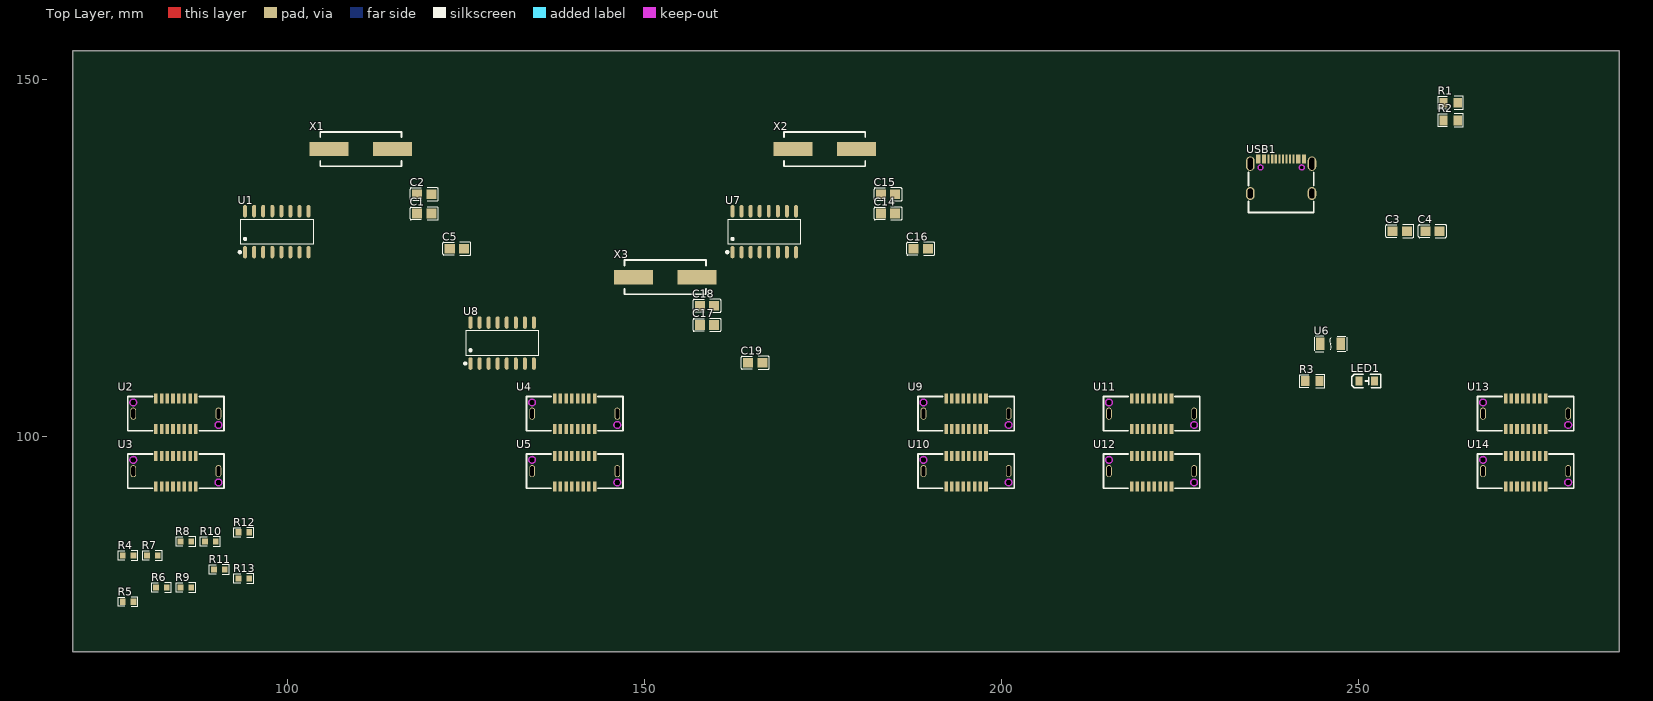
[diagram p0: Top Layer view]
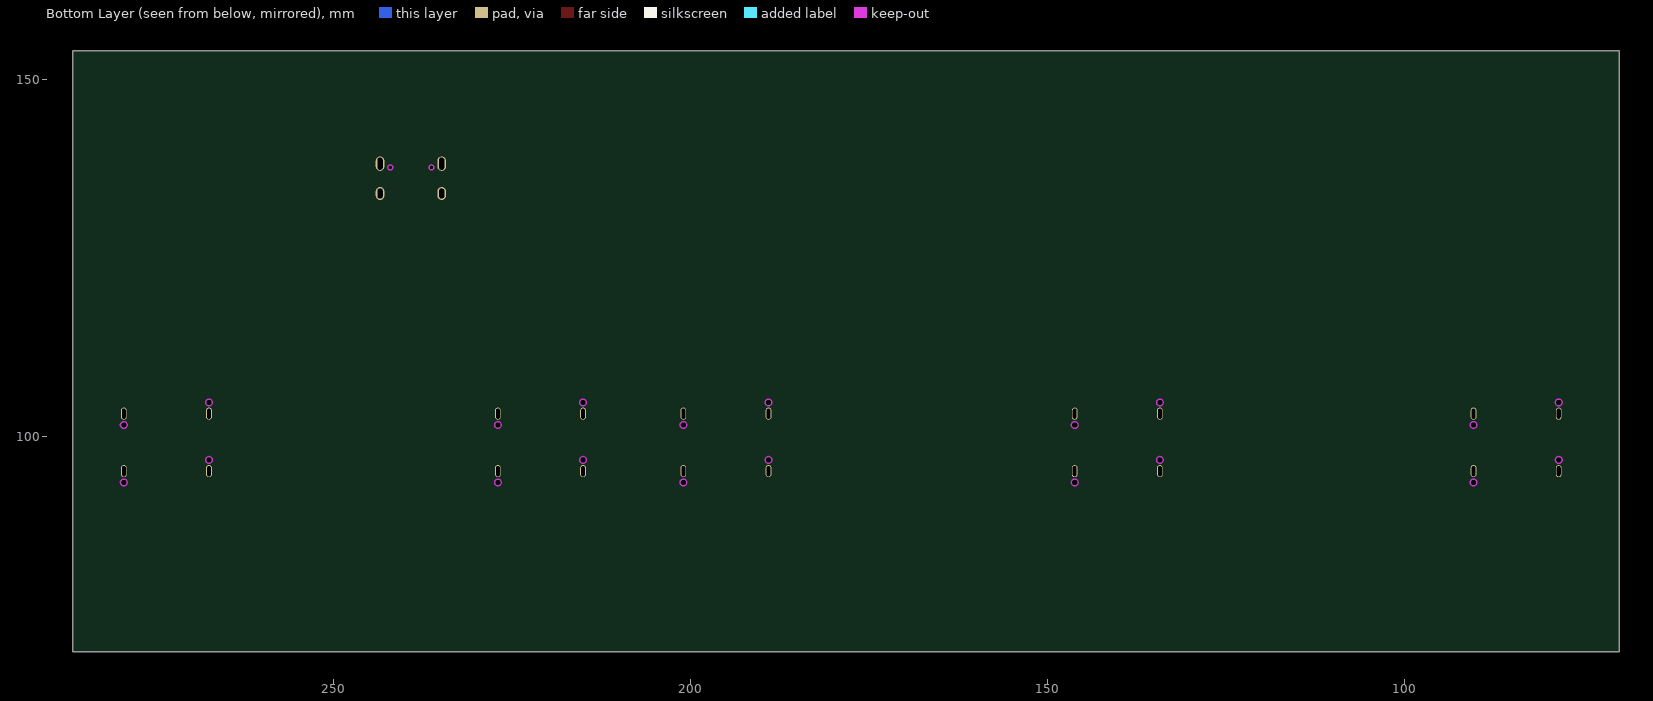
[diagram p1: Bottom Layer view, seen from below]
# Altium PCB MISC51596.pcbdoc
Units mm, origin at the board's own origin, x right, y up, seen from the top; angles counter-clockwise.
Board outline 216.76 x 84.23 mm, 2 copper layers (Top Layer, Bottom Layer), stack 1.58 mm thick; 43 components, 45 nets, 306 pads, 0 vias.

## Layer stack, top to bottom
Top Solder Mask Layer: solder mask 0.01, Dk 3.3
Top Layer: signal copper 0.035
Dielectric1: surface 1.51, FR4, Dk 4.5
Bottom Layer: signal copper 0.035
Bottom Solder Mask Layer: solder mask 0.01, Dk 3.3

## Board outline
286.61,69.85 69.85,69.85 69.85,154.083 286.61,154.083

## Design rules (kind name [scope] priority, off if disabled: settings)
BoardOutlineClearance copperThickness2oz_1 [All] p2 off: genericclearance=0.203 ignorepadtopadclearanceinfootprint=FALSE except(0: Arc-SplitContinuation Track-SplitContinuation SMDPad-SplitContinuation THPad-SplitContinuation Via-SplitContinuation Fill-SplitContinuation Region-SplitContinuation Poly-SplitContinuation Text-SplitContinuation Hole-SplitContinuation; 0.152: SMDPad-CutoutEdge THPad-CutoutEdge Via-CutoutEdge Fill-CutoutEdge Region-CutoutEdge Text-CutoutEdge Hole-CutoutEdge; 0.254: Poly-OutlineEdge Poly-CutoutEdge; 0.3: Arc-OutlineEdge Track-OutlineEdge SMDPad-OutlineEdge THPad-OutlineEdge Via-OutlineEdge Fill-OutlineEdge Region-OutlineEdge Text-OutlineEdge Hole-OutlineEdge Arc-CutoutEdge Track-CutoutEdge)
BoardOutlineClearance Plane_innerPlane_1 [All] p4 off: genericclearance=0.102 ignorepadtopadclearanceinfootprint=FALSE except(0: Arc-SplitContinuation Track-SplitContinuation SMDPad-SplitContinuation THPad-SplitContinuation Via-SplitContinuation Fill-SplitContinuation Region-SplitContinuation Poly-SplitContinuation Text-SplitContinuation Hole-SplitContinuation; 0.152: SMDPad-CutoutEdge THPad-CutoutEdge Via-CutoutEdge Fill-CutoutEdge Region-CutoutEdge Text-CutoutEdge Hole-CutoutEdge; 0.254: Poly-OutlineEdge Poly-CutoutEdge; 0.3: Arc-OutlineEdge Track-OutlineEdge SMDPad-OutlineEdge THPad-OutlineEdge Via-OutlineEdge Fill-OutlineEdge Region-OutlineEdge Text-OutlineEdge Hole-OutlineEdge Arc-CutoutEdge Track-CutoutEdge)
BoardOutlineClearance Copper_copperRegion_1 [All] p6 off: genericclearance=0.102 ignorepadtopadclearanceinfootprint=FALSE except(0: Arc-SplitContinuation Track-SplitContinuation SMDPad-SplitContinuation THPad-SplitContinuation Via-SplitContinuation Fill-SplitContinuation Region-SplitContinuation Poly-SplitContinuation Text-SplitContinuation Hole-SplitContinuation; 0.152: SMDPad-CutoutEdge THPad-CutoutEdge Via-CutoutEdge Fill-CutoutEdge Region-CutoutEdge Text-CutoutEdge Hole-CutoutEdge; 0.254: Poly-OutlineEdge Poly-CutoutEdge; 0.3: Arc-OutlineEdge Track-OutlineEdge SMDPad-OutlineEdge THPad-OutlineEdge Via-OutlineEdge Fill-OutlineEdge Region-OutlineEdge Text-OutlineEdge Hole-OutlineEdge Arc-CutoutEdge Track-CutoutEdge)
BoardOutlineClearance copperThickness1oz_1 [All] p8: genericclearance=0.102 ignorepadtopadclearanceinfootprint=FALSE except(0: Arc-SplitContinuation Track-SplitContinuation SMDPad-SplitContinuation THPad-SplitContinuation Via-SplitContinuation Fill-SplitContinuation Region-SplitContinuation Poly-SplitContinuation Text-SplitContinuation Hole-SplitContinuation; 0.152: SMDPad-CutoutEdge THPad-CutoutEdge Via-CutoutEdge Fill-CutoutEdge Region-CutoutEdge Text-CutoutEdge Hole-CutoutEdge; 0.254: Poly-OutlineEdge Poly-CutoutEdge; 0.3: Arc-OutlineEdge Track-OutlineEdge SMDPad-OutlineEdge THPad-OutlineEdge Via-OutlineEdge Fill-OutlineEdge Region-OutlineEdge Text-OutlineEdge Hole-OutlineEdge Arc-CutoutEdge Track-CutoutEdge)
Clearance copperThickness2oz [All] p1 off: gap=0.203 ignorepadtopadclearanceinfootprint=FALSE except(0.152: SMDPad-Track SMDPad-SMDPad THPad-Track SMDPad-THPad THPad-THPad Track-Via SMDPad-Via THPad-Via Via-Via Fill-Track Region-Track Fill-SMDPad Region-SMDPad Fill-THPad Region-THPad Fill-Via Region-Via Fill-Fill Fill-Region Region-Region Arc-Track Arc-SMDPad Arc-THPad Arc-Via Fill-Arc Region-Arc Arc-Arc Text-Track SMDPad-Text Text-THPad Text-Via Fill-Text Region-Text Arc-Text Text-Text Hole-Track Hole-SMDPad Hole-THPad Hole-Via Fill-Hole Region-Hole Hole-Arc Hole-Text; 0.254: Poly-Track Poly-SMDPad Poly-THPad Poly-Via Poly-Fill Poly-Region Poly-Poly Poly-Arc Poly-Text Poly-Hole)
Clearance Plane_innerPlane [All] p3 off: gap=0.102 ignorepadtopadclearanceinfootprint=FALSE except(0.152: SMDPad-Track SMDPad-SMDPad THPad-Track SMDPad-THPad THPad-THPad Track-Via SMDPad-Via THPad-Via Via-Via Fill-Track Region-Track Fill-SMDPad Region-SMDPad Fill-THPad Region-THPad Fill-Via Region-Via Fill-Fill Fill-Region Region-Region Arc-Track Arc-SMDPad Arc-THPad Arc-Via Fill-Arc Region-Arc Arc-Arc Text-Track SMDPad-Text Text-THPad Text-Via Fill-Text Region-Text Arc-Text Text-Text Hole-Track Hole-SMDPad Hole-THPad Hole-Via Fill-Hole Region-Hole Hole-Arc Hole-Text; 0.254: Poly-Track Poly-SMDPad Poly-THPad Poly-Via Poly-Fill Poly-Region Poly-Poly Poly-Arc Poly-Text Poly-Hole)
Clearance Copper_copperRegion [All] p5 off: gap=0.102 ignorepadtopadclearanceinfootprint=FALSE except(0.152: SMDPad-Track SMDPad-SMDPad THPad-Track SMDPad-THPad THPad-THPad Track-Via SMDPad-Via THPad-Via Via-Via Fill-Track Region-Track Fill-SMDPad Region-SMDPad Fill-THPad Region-THPad Fill-Via Region-Via Fill-Fill Fill-Region Region-Region Arc-Track Arc-SMDPad Arc-THPad Arc-Via Fill-Arc Region-Arc Arc-Arc Text-Track SMDPad-Text Text-THPad Text-Via Fill-Text Region-Text Arc-Text Text-Text Hole-Track Hole-SMDPad Hole-THPad Hole-Via Fill-Hole Region-Hole Hole-Arc Hole-Text; 0.254: Poly-Track Poly-SMDPad Poly-THPad Poly-Via Poly-Fill Poly-Region Poly-Poly Poly-Arc Poly-Text Poly-Hole)
Clearance copperThickness1oz [All] p7: gap=0.102 ignorepadtopadclearanceinfootprint=FALSE except(0.152: SMDPad-Track SMDPad-SMDPad THPad-Track SMDPad-THPad THPad-THPad Track-Via SMDPad-Via THPad-Via Via-Via Fill-Track Region-Track Fill-SMDPad Region-SMDPad Fill-THPad Region-THPad Fill-Via Region-Via Fill-Fill Fill-Region Region-Region Arc-Track Arc-SMDPad Arc-THPad Arc-Via Fill-Arc Region-Arc Arc-Arc Text-Track SMDPad-Text Text-THPad Text-Via Fill-Text Region-Text Arc-Text Text-Text Hole-Track Hole-SMDPad Hole-THPad Hole-Via Fill-Hole Region-Hole Hole-Arc Hole-Text; 0.254: Poly-Track Poly-SMDPad Poly-THPad Poly-Via Poly-Fill Poly-Region Poly-Poly Poly-Arc Poly-Text Poly-Hole)
DiffPairsRouting differentialPair [All] p1: maxlimit=0.152 minlimit=0.152 mostfreqgap=0.152 toplayer_minwidth=0.127 toplayer_prefwidth=0.254 toplayer_maxwidth=2.54 toplayer_mingap=0.152 toplayer_prefgap=0.152 toplayer_maxgap=0.152 bottomlayer_minwidth=0.127 bottomlayer_prefwidth=0.254 bottomlayer_maxwidth=2.54 bottomlayer_mingap=0.152 bottomlayer_prefgap=0.152 bottomlayer_maxgap=0.152 maxuncoupledlength=0.127
HoleToHoleClearance otherClearance [All] p1: gap=0.3 allowstackedmicrovias=TRUE
Length netLength [All] p1: minlimit=0 maxlimit=0
PasteMaskExpansion pasteMaskExpansion [All] p1: expansion=0
PlaneConnect innerPlane [All] p1: planeconnectstyle=Relief reliefexpansion=0.508 reliefentries=4 reliefconductorwidth=0.254 reliefairgap=0.254
PolygonConnect copperRegion [All] p1: connectstyle=Relief reliefconductorwidth=0.254 reliefentries=4 polygonreliefangle="90 Angle" airgapwidth=0.254 via.connectstyle=Relief via.reliefconductorwidth=0.254 via.reliefentries=4 via.polygonreliefangle="90 Angle" via.airgapwidth=0.254
RoutingVias viaSize [All] p1: holewidth=0.305 width=0.61 viastyle="Through Hole" minholewidth=0.3 minwidth=0.5 maxholewidth=6.299 maxwidth=10
SolderMaskExpansion solderMaskExpansion [IsVia] p1: expansion=-25.4 istentingtop=TRUE
SolderMaskExpansion solderMaskExpansion [All] p2: expansion=0.051 istentingtop=FALSE
Width copperThickness2oz_2 [All] p1 off: maxlimit=2.54 minlimit=0.203 preferedwidth=0.254
Width copperThickness1oz_2 [All] p2: maxlimit=2.54 minlimit=0.127 preferedwidth=0.254

## Components (designator, comment, footprint, x,y, rotation, side; value= is the part's Value field where it differs from the comment)
C1 "100nF" C0805 119.111,131.274 r0 top
C2 "100nF" C0805 119.111,133.959 r0 top
C3 "10UF" C0805 255.864,128.815 r0 top
C4 "0.1UF" C0805 260.443,128.815 r0 top
C5 "0.1UF" C0805 123.69,126.355 r0 top
C14 "100nF" C0805 184.127,131.274 r0 top
C15 "100nF" C0805 184.127,133.959 r0 top
C16 "0.1UF" C0805 188.706,126.355 r0 top
C17 "100nF" C0805 158.75,115.657 r0 top
C18 "100nF" C0805 158.75,118.342 r0 top
C19 "0.1UF" C0805 165.497,110.36 r0 top
LED1 "" LED_0805 251.267,107.788 r0 top
R1 "5.1K" R0805 262.983,146.816 r0 top
R2 "5.1K" R0805 262.983,144.329 r0 top
R3 "2K" R0805 243.605,107.788 r0 top
R4 "10K" R0603 77.585,83.348 r0 top
R5 "10K" R0603 77.585,76.861 r0 top
R6 "10K" R0603 82.278,78.834 r0 top
R7 "10K" R0603 81.008,83.348 r0 top
R8 "10K" R0603 85.7,85.321 r0 top
R9 "10K" R0603 85.7,78.834 r0 top
R10 "10K" R0603 89.123,85.321 r0 top
R11 "10K" R0603 90.393,81.374 r0 top
R12 "10K" R0603 93.815,86.591 r0 top
R13 "10K" R0603 93.815,80.104 r0 top
U1 "SL2.1A" SOP-16_L10.0-W3.9-P1.27-LS6.0-BL 98.441,128.734 r0 top
U2 "EZ-USBC-1143C" USB-SMD_EZ-USBC-1143C 84.294,103.217 r0 top
U3 "EZ-USBC-1143C" USB-SMD_EZ-USBC-1143C 84.294,95.163 r0 top
U4 "EZ-USBC-1143C" USB-SMD_EZ-USBC-1143C 140.2,103.217 r0 top
U5 "EZ-USBC-1143C" USB-SMD_EZ-USBC-1143C 140.2,95.163 r0 top
U6 "1.5A快恢复保险丝-1206" F1206 246.145,113.008 r0 top
U7 "SL2.1A" SOP-16_L10.0-W3.9-P1.27-LS6.0-BL 166.767,128.734 r0 top
U8 "SL2.1A" SOP-16_L10.0-W3.9-P1.27-LS6.0-BL 130.04,113.117 r0 top
U9 "EZ-USBC-1143C" USB-SMD_EZ-USBC-1143C 195.056,103.217 r0 top
U10 "EZ-USBC-1143C" USB-SMD_EZ-USBC-1143C 195.056,95.163 r0 top
U11 "EZ-USBC-1143C" USB-SMD_EZ-USBC-1143C 221.056,103.217 r0 top
U12 "EZ-USBC-1143C" USB-SMD_EZ-USBC-1143C 221.056,95.163 r0 top
U13 "EZ-USBC-1143C" USB-SMD_EZ-USBC-1143C 273.49,103.217 r0 top
U14 "EZ-USBC-1143C" USB-SMD_EZ-USBC-1143C 273.49,95.163 r0 top
USB1 "typec" USB-C-SMD_KH-TYPE-C-16P 239.228,136.499 r0 top
X1 "12MHz" CRYSTAL-SMD_L11.1-W4.8-LS12.3 110.221,140.309 r0 top
X2 "12MHz" CRYSTAL-SMD_L11.1-W4.8-LS12.3 175.237,140.309 r0 top
X3 "12MHz" CRYSTAL-SMD_L11.1-W4.8-LS12.3 152.9,122.348 r0 top

## Footprints (in the part's own frame and the unit in brackets; to place one, negate y for a bottom-side part, rotate by r counter-clockwise, add the part's x,y. Pads: shape width x height; smd on the part's side, far side on the other; paste and mask are expansions set on the pad)
C0805 [mm]
  rect 1.41x1.35 smd paste-100 mask+0.051: 1(-1,0) 2(1,0)
  silkscreen extent -1.96,-0.9 1.96,0.9
CRYSTAL-SMD_L11.1-W4.8-LS12.3 [mm]
  rect 5.5x2 smd: 1(-4.45,0) 2(4.45,0)
  silkscreen extent -5.7,-2.4 5.7,2.4
F1206 [mm]
  rect 1.19x1.728 smd: 1(-1.445,0) 2(1.445,0)
  silkscreen extent -2.27,-1.09 2.27,1.09
LED_0805 [mm]
  rect 1x1.25 smd paste+0 mask+0.051: 1(-1.15,0.005) 2(1.05,0.005)
  silkscreen extent -2.15,-0.94 1.93,0.97
R0603 [mm]
  rect 0.806x0.864 smd paste-100 mask+0.051: 1(-0.753,0) 2(0.753,0)
  silkscreen extent -1.39,-0.66 1.39,0.66
R0805 [mm]
  rect 1.133x1.377 smd paste-100 mask+0.051: 1(-1,0) 2(1,0)
  silkscreen extent -1.76,-0.92 1.76,0.92
SOP-16_L10.0-W3.9-P1.27-LS6.0-BL [mm]
  oval 0.56x1.745 smd: 1(-4.445,-2.872) 2(-3.175,-2.872) 3(-1.905,-2.872) 4(-0.635,-2.872) 5(0.635,-2.872) 6(1.905,-2.872) 7(3.175,-2.872) 8(4.445,-2.872) 9(4.445,2.872) 10(3.175,2.872) 11(1.905,2.872) 12(0.635,2.872) 13(-0.635,2.872) 14(-1.905,2.872) 15(-3.175,2.872) 16(-4.445,2.872)
  silkscreen extent -5.33,-3.02 5.08,1.77
USB-C-SMD_KH-TYPE-C-16P [mm]
  oval 1.2x2 hole 0.7 slot 1.7 at 90 deg: 1(-4.32,1.765) 2(4.32,1.765)
  oval 1.2x1.8 hole 0.7 slot 1.4 at 90 deg: 3(-4.32,-2.415) 4(4.32,-2.415)
  rect 0.3x1.3 smd paste-100 mask+0.05: A1(-3.35,2.415) A4(-2.55,2.415) A5(-1.25,2.415) A6(-0.25,2.415) A7(0.25,2.415) A8(1.25,2.415) A9(2.55,2.415) A12(3.35,2.415) B1(3.05,2.415) B4(2.25,2.415) B5(1.75,2.415) B6(0.75,2.415) B7(-0.75,2.415) B8(-1.75,2.415) B9(-2.25,2.415) B12(-3.05,2.415)
  Board Outline Layer circle w0.003: c-2.89,1.235 r0.35
  Board Outline Layer circle w0.003: c2.89,1.235 r0.35
  Board Outline Layer region: -2.54,1.235 -2.575,1.083 -2.672,0.961 -2.812,0.894 -2.968,0.894 -3.108,0.961 -3.205,1.083 -3.24,1.235 -3.24,1.235 -3.205,1.387 -3.108,1.509 -2.968,1.576 -2.812,1.576 -2.672,1.509 -2.575,1.387 -2.54,1.235
  Board Outline Layer region: -2.54,1.235 -2.549,1.157 -2.575,1.083 -2.616,1.017 -2.672,0.961 -2.738,0.92 -2.812,0.894 -2.89,0.885 -2.968,0.894 -3.042,0.92 -3.108,0.961 -3.164,1.017 -3.205,1.083 -3.231,1.157 -3.24,1.235 -3.231,1.313 -3.205,1.387 -3.164,1.453 -3.108,1.509 -3.042,1.55 -2.968,1.576 -2.89,1.585 -2.812,1.576 -2.738,1.55 -2.672,1.509 -2.616,1.453 -2.575,1.387 -2.549,1.313
  Board Outline Layer region: 3.24,1.235 3.205,1.083 3.108,0.961 2.968,0.894 2.812,0.894 2.672,0.961 2.575,1.083 2.54,1.235 2.54,1.235 2.575,1.387 2.672,1.509 2.812,1.576 2.968,1.576 3.108,1.509 3.205,1.387 3.24,1.235
  Board Outline Layer region: 3.24,1.235 3.231,1.157 3.205,1.083 3.164,1.017 3.108,0.961 3.042,0.92 2.968,0.894 2.89,0.885 2.812,0.894 2.738,0.92 2.672,0.961 2.616,1.017 2.575,1.083 2.549,1.157 2.54,1.235 2.549,1.313 2.575,1.387 2.616,1.453 2.672,1.509 2.738,1.55 2.812,1.576 2.89,1.585 2.968,1.576 3.042,1.55 3.108,1.509 3.164,1.453 3.205,1.387 3.231,1.313
  Multi-Layer board cut-out: -2.54,1.235 -2.575,1.083 -2.672,0.961 -2.812,0.894 -2.968,0.894 -3.108,0.961 -3.205,1.083 -3.24,1.235 -3.24,1.235 -3.205,1.387 -3.108,1.509 -2.968,1.576 -2.812,1.576 -2.672,1.509 -2.575,1.387 -2.54,1.235
  Multi-Layer board cut-out: 3.24,1.235 3.205,1.083 3.108,0.961 2.968,0.894 2.812,0.894 2.672,0.961 2.575,1.083 2.54,1.235 2.54,1.235 2.575,1.387 2.672,1.509 2.812,1.576 2.968,1.576 3.108,1.509 3.205,1.387 3.24,1.235
  silkscreen extent -4.57,-5.08 4.57,0.57
USB-SMD_EZ-USBC-1143C [mm]
  oval 0.8x1.7 hole 0.5 slot 1.4 at 90 deg paste+0 mask+0.05: 17(-5.97,0) 18(5.97,0)
  rect 0.5x1.4 smd paste-100 mask+0.05: A1(-2.8,2.13) A4(-2,2.13) A5(-1.2,2.13) A6(-0.4,2.13) A7(0.4,2.13) A8(1.2,2.13) A9(2,2.13) A12(2.8,2.13) B1(2.8,-2.13) B4(2,-2.13) B5(1.2,-2.13) B6(0.4,-2.13) B7(-0.4,-2.13) B8(-1.2,-2.13) B9(-2,-2.13) B12(-2.8,-2.13)
  Board Outline Layer circle w0.003: c-5.97,1.58 r0.475
  Board Outline Layer circle w0.003: c5.97,-1.58 r0.475
  Board Outline Layer region: -5.495,1.58 -5.542,1.374 -5.674,1.209 -5.864,1.117 -6.076,1.117 -6.266,1.209 -6.398,1.374 -6.445,1.58 -6.445,1.58 -6.398,1.786 -6.266,1.951 -6.076,2.043 -5.864,2.043 -5.674,1.951 -5.542,1.786 -5.495,1.58
  Board Outline Layer region: -5.495,1.58 -5.504,1.487 -5.531,1.398 -5.575,1.316 -5.634,1.244 -5.706,1.185 -5.788,1.141 -5.877,1.114 -5.97,1.105 -6.063,1.114 -6.152,1.141 -6.234,1.185 -6.306,1.244 -6.365,1.316 -6.409,1.398 -6.436,1.487 -6.445,1.58 -6.436,1.673 -6.409,1.762 -6.365,1.844 -6.306,1.916 -6.234,1.975 -6.152,2.019 -6.063,2.046 -5.97,2.055 -5.877,2.046 -5.788,2.019 -5.706,1.975 -5.634,1.916 -5.575,1.844 -5.531,1.762 -5.504,1.673
  Board Outline Layer region: 6.445,-1.58 6.398,-1.786 6.266,-1.951 6.076,-2.043 5.864,-2.043 5.674,-1.951 5.542,-1.786 5.495,-1.58 5.495,-1.58 5.542,-1.374 5.674,-1.209 5.864,-1.117 6.076,-1.117 6.266,-1.209 6.398,-1.374 6.445,-1.58
  Board Outline Layer region: 6.445,-1.58 6.436,-1.673 6.409,-1.762 6.365,-1.844 6.306,-1.916 6.234,-1.975 6.152,-2.019 6.063,-2.046 5.97,-2.055 5.877,-2.046 5.788,-2.019 5.706,-1.975 5.634,-1.916 5.575,-1.844 5.531,-1.762 5.504,-1.673 5.495,-1.58 5.504,-1.487 5.531,-1.398 5.575,-1.316 5.634,-1.244 5.706,-1.185 5.788,-1.141 5.877,-1.114 5.97,-1.105 6.063,-1.114 6.152,-1.141 6.234,-1.185 6.306,-1.244 6.365,-1.316 6.409,-1.398 6.436,-1.487
  Multi-Layer board cut-out: -5.495,1.58 -5.542,1.374 -5.674,1.209 -5.864,1.117 -6.076,1.117 -6.266,1.209 -6.398,1.374 -6.445,1.58 -6.445,1.58 -6.398,1.786 -6.266,1.951 -6.076,2.043 -5.864,2.043 -5.674,1.951 -5.542,1.786 -5.495,1.58
  Multi-Layer board cut-out: 6.445,-1.58 6.398,-1.786 6.266,-1.951 6.076,-2.043 5.864,-2.043 5.674,-1.951 5.542,-1.786 5.495,-1.58 5.495,-1.58 5.542,-1.374 5.674,-1.209 5.864,-1.117 6.076,-1.117 6.266,-1.209 6.398,-1.374 6.445,-1.58
  silkscreen extent -6.75,-2.4 6.75,2.4

## Nets (pads, with @x,y where several pads share a name; then routed paths per layer and width w, separated by ;. In a path a pad name is that pad's centre, name@x,y a point inside that pad or via, vN(x,y) a via of type N, cw(c..) or ccw(c..) an arc to the next point about the centre after c; other vN are vias at no path point)
$1N748: C2.1 U1.14
$1N752: C1.1 U1.13
$1N850: U1.15 X1.1
$1N854: U1.16 X1.2
$1N2453: LED1.2 R3.1
$1N2514: U7.16 X2.2
$1N2515: U7.15 X2.1
$1N2516: C14.1 U7.13
$1N2517: C15.1 U7.14
$1N2531: U8.16 X3.2
$1N2532: U8.15 X3.1
$1N2533: C17.1 U8.13
$1N2534: C18.1 U8.14
+5V: C5.2 C16.2 C19.2 R4.1 R5.1 R6.1 R7.1 R8.1 R9.1 R10.1 R11.1 R12.1 R13.1 U1.11 U2.A4 U2.A9 U2.B4 U2.B9 U3.A4 U3.A9 U3.B4 U3.B9 U4.A4 U4.A9 U4.B4 U4.B9 U5.A4 U5.A9 U5.B4 U5.B9 U7.11 U8.11 U9.A4 U9.A9 U9.B4 U9.B9 U10.A4 U10.A9 U10.B4 U10.B9 U11.A4 U11.A9 U11.B4 U11.B9 U12.A4 U12.A9 U12.B4 U12.B9 U13.A4 U13.A9 U13.B4 U13.B9 U14.A4 U14.A9 U14.B4 U14.B9
CC1: R2.1 USB1.A5
CC2: R1.1 USB1.B5
DM: U1.9 USB1.A7 USB1.B7
DM1: U1.3 U2.A7 U2.B7
DM2: U1.1 U3.A7 U3.B7
DM3: U4.A7 U4.B7 U7.7
DM4: U5.A7 U5.B7 U7.5
DM5: U7.3 U9.A7 U9.B7
DM6: U7.1 U10.A7 U10.B7
DM7: U8.7 U11.A7 U11.B7
DM8: U8.5 U12.A7 U12.B7
DM9: U8.3 U13.A7 U13.B7
DM10: U8.1 U14.A7 U14.B7
DM11: U1.7 U7.9
DM22: U1.5 U8.9
DP: U1.10 USB1.A6 USB1.B6
DP1: U1.4 U2.A6 U2.B6
DP2: U1.2 U3.A6 U3.B6
DP3: U4.A6 U4.B6 U7.8
DP4: U5.A6 U5.B6 U7.6
DP5: U7.4 U9.A6 U9.B6
DP6: U7.2 U10.A6 U10.B6
DP7: U8.8 U11.A6 U11.B6
DP8: U8.6 U12.A6 U12.B6
DP9: U8.4 U13.A6 U13.B6
DP10: U8.2 U14.A6 U14.B6
DP11: U1.8 U7.10
DP22: U1.6 U8.10
GND: C1.2 C2.2 C3.1 C4.1 C5.1 C14.2 C15.2 C16.1 C17.2 C18.2 C19.1 LED1.1 R1.2 R2.2 R4.2 R5.2 R6.2 R7.2 R8.2 R9.2 R10.2 R11.2 R12.2 R13.2 U1.12 U2.17 U2.18 U2.A1 U2.A12 U2.B1 U2.B12 U3.17 U3.18 U3.A1 U3.A12 U3.B1 U3.B12 U4.17 U4.18 U4.A1 U4.A12 U4.B1 U4.B12 U5.17 U5.18 U5.A1 U5.A12 U5.B1 U5.B12 U7.12 U8.12 U9.17 U9.18 U9.A1 U9.A12 U9.B1 U9.B12 U10.17 U10.18 U10.A1 U10.A12 U10.B1 U10.B12 U11.17 U11.18 U11.A1 U11.A12 U11.B1 U11.B12 U12.17 U12.18 U12.A1 U12.A12 U12.B1 U12.B12 U13.17 U13.18 U13.A1 U13.A12 U13.B1 U13.B12 U14.17 U14.18 U14.A1 U14.A12 U14.B1 U14.B12 USB1.1 USB1.2 USB1.3 USB1.4 USB1.A1 USB1.A12 USB1.B1 USB1.B12
VCC: R3.2 U6.2
VCC+5V: C3.2 C4.2 U6.1 USB1.A4 USB1.A9 USB1.B4 USB1.B9
pads on no net: U2.A5 U2.A8 U2.B5 U2.B8 U3.A5 U3.A8 U3.B5 U3.B8 U4.A5 U4.A8 U4.B5 U4.B8 U5.A5 U5.A8 U5.B5 U5.B8 U9.A5 U9.A8 U9.B5 U9.B8 U10.A5 U10.A8 U10.B5 U10.B8 U11.A5 U11.A8 U11.B5 U11.B8 U12.A5 U12.A8 U12.B5 U12.B8 U13.A5 U13.A8 U13.B5 U13.B8 U14.A5 U14.A8 U14.B5 U14.B8 USB1.A8 USB1.B8